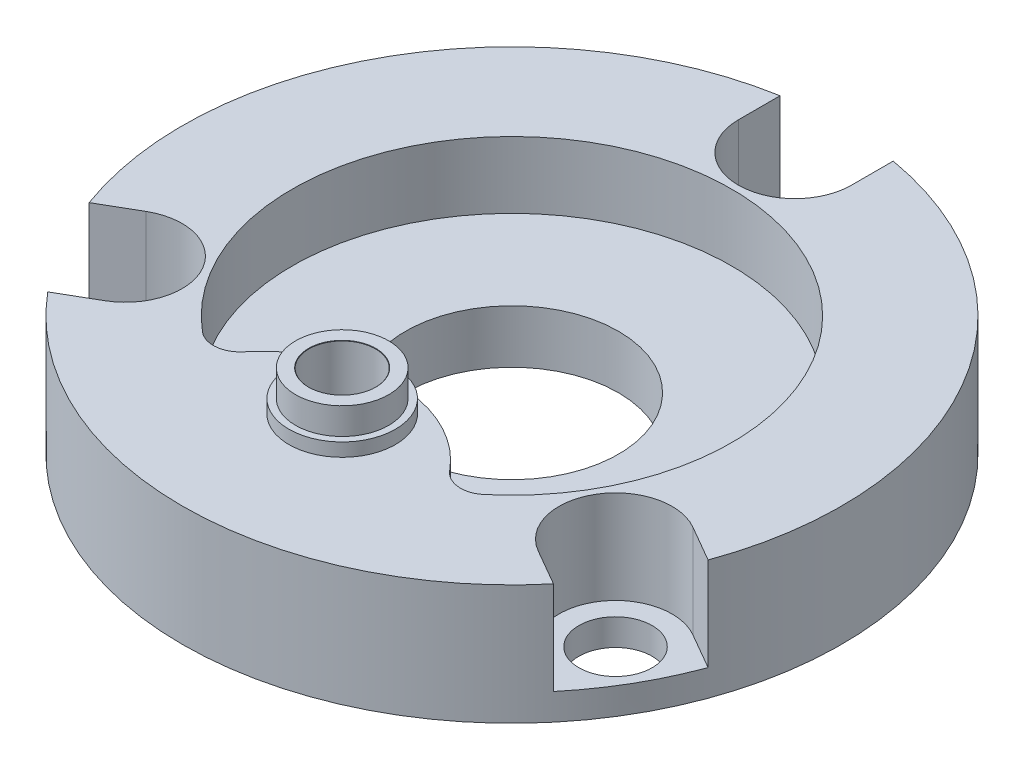
from build123d import *

# Parameters (mm, degrees)
SKETCH1_R                              = 24.75
BOSS_EXTRUDE1_DEPTH                    = 9
CUT_EXTRUDE1_START                     = -7
CUT_EXTRUDE1_DEPTH                     = 44.140351409
SKETCH3_R                              = 2.75
CUT_EXTRUDE2_DEPTH                     = 7
CIRPATTERN1_COUNT                      = 3
SKETCH5_R                              = 4
BOSS_EXTRUDE2_DEPTH                    = 1
SKETCH6_R                              = 3.5
BOSS_EXTRUDE3_DEPTH                    = 3
F_5_0MM_BLIND_DOWEL_HOLE_1_D           = 5
F_5_0MM_BLIND_DOWEL_HOLE_1_DEPTH       = 5
F_5_0MM_BLIND_DOWEL_HOLE_1_CSINK_D     = 5.05
F_5_0MM_BLIND_DOWEL_HOLE_1_CSINK_ANGLE = 90
F_5_0MM_BLIND_DOWEL_HOLE_1_TIP         = 1.502151548
CUT_EXTRUDE3_START                     = 7
CUT_EXTRUDE3_DEPTH                     = 5
SKETCH9_R                              = 8
CUT_EXTRUDE4_DEPTH                     = 5


with BuildPart() as part:
    # Sketch1 → Boss-Extrude1 (new body)
    with BuildSketch(Plane(origin=(0, 0, 0), x_dir=(1, 0, 0), z_dir=(0, 1, 0))):
        with Locations(Location((0, 0, 0), (0, 0, 270))):
            Circle(SKETCH1_R)
    extrude(amount=BOSS_EXTRUDE1_DEPTH)

    # Sketch2 → Cut-Extrude1 (cut)
    with BuildSketch(Plane(origin=(0, 9, 0), x_dir=(1, 0, 0), z_dir=(0, 1, 0)).offset(CUT_EXTRUDE1_START)):
        with BuildLine():
            Line((-4.25, 21.25), (-4.25, 27.920433859))
            Line((-4.25, 27.920433859), (4.25, 27.920433859))
            Line((4.25, 27.920433859), (4.25, 21.25))
            ThreePointArc((4.25, 21.25), (0, 17), (-4.25, 21.25))
        make_face()
    cut_extrude1 = extrude(amount=CUT_EXTRUDE1_DEPTH, mode=Mode.SUBTRACT)

    # Sketch3 → Cut-Extrude2 (cut)
    with BuildSketch(Plane(origin=(0, 2, 0), x_dir=(1, 0, 0), z_dir=(0, 1, 0))):
        with Locations(Location((0, 21.25, 0), (0, 0, 270))):
            Circle(SKETCH3_R)
    cut_extrude2 = extrude(amount=-CUT_EXTRUDE2_DEPTH, mode=Mode.SUBTRACT)

    # CirPattern1: Cut-Extrude1, Cut-Extrude2 ×3 about axis
    cirpattern1_axis = Axis((0, 0, 0), (0, 1, 0))
    add([cut_extrude1.rotate(cirpattern1_axis, i * 360 / CIRPATTERN1_COUNT) for i in range(1, CIRPATTERN1_COUNT)], mode=Mode.SUBTRACT)
    add([cut_extrude2.rotate(cirpattern1_axis, i * 360 / CIRPATTERN1_COUNT) for i in range(1, CIRPATTERN1_COUNT)], mode=Mode.SUBTRACT)

    # Sketch5 → Boss-Extrude2 (add)
    with BuildSketch(Plane(origin=(0, 9, 0), x_dir=(1, 0, 0), z_dir=(0, 1, 0))):
        with Locations(Location((0, -12.75, 0), (0, 0, 270))):
            Circle(SKETCH5_R)
    extrude(amount=BOSS_EXTRUDE2_DEPTH)

    # Sketch6 → Boss-Extrude3 (add)
    with BuildSketch(Plane(origin=(0, 9, 0), x_dir=(1, 0, 0), z_dir=(0, 1, 0))):
        with Locations(Location((0, -12.75, 0), (0, 0, 270))):
            Circle(SKETCH6_R)
    extrude(amount=BOSS_EXTRUDE3_DEPTH)

    # Ø5.0mm blind dowel hole 1
    with Locations(Plane(origin=(0, 12, 0), x_dir=(1, 0, 0), z_dir=(0, 1, 0))):
        with Locations((0, -12.75)):
            CounterSinkHole(F_5_0MM_BLIND_DOWEL_HOLE_1_D / 2, F_5_0MM_BLIND_DOWEL_HOLE_1_CSINK_D / 2, depth=F_5_0MM_BLIND_DOWEL_HOLE_1_DEPTH, counter_sink_angle=F_5_0MM_BLIND_DOWEL_HOLE_1_CSINK_ANGLE)
            with Locations((0, 0, -(F_5_0MM_BLIND_DOWEL_HOLE_1_DEPTH + F_5_0MM_BLIND_DOWEL_HOLE_1_TIP / 2))):  # 118° drill point
                Cone(0, F_5_0MM_BLIND_DOWEL_HOLE_1_D / 2, F_5_0MM_BLIND_DOWEL_HOLE_1_TIP, mode=Mode.SUBTRACT)

    # Sketch4 → Cut-Extrude3 (cut)
    with BuildSketch(Plane(origin=(0, 2, 0), x_dir=(1, 0, 0), z_dir=(0, 1, 0)).offset(CUT_EXTRUDE3_START)):
        with BuildLine():
            ThreePointArc((10.559685096, -12.678448276), (0, 16.5), (-10.559685096, -12.678448276))
            ThreePointArc((-10.559685096, -12.678448276), (-9.090434755, -13.132688982), (-7.733102721, -12.409722222))
            ThreePointArc((-7.733102721, -12.409722222), (0, -8.75), (7.733102721, -12.409722222))
            ThreePointArc((7.733102721, -12.409722222), (9.090434755, -13.132688982), (10.559685096, -12.678448276))
        make_face()
    extrude(amount=-CUT_EXTRUDE3_DEPTH, mode=Mode.SUBTRACT)

    # Sketch9 → Cut-Extrude4 (cut)
    with BuildSketch(Plane.XZ):
        with Locations(Location((0, 0, 0), (0, 0, 270))):
            Circle(SKETCH9_R)
    extrude(amount=-CUT_EXTRUDE4_DEPTH, mode=Mode.SUBTRACT)


solid = part.part
